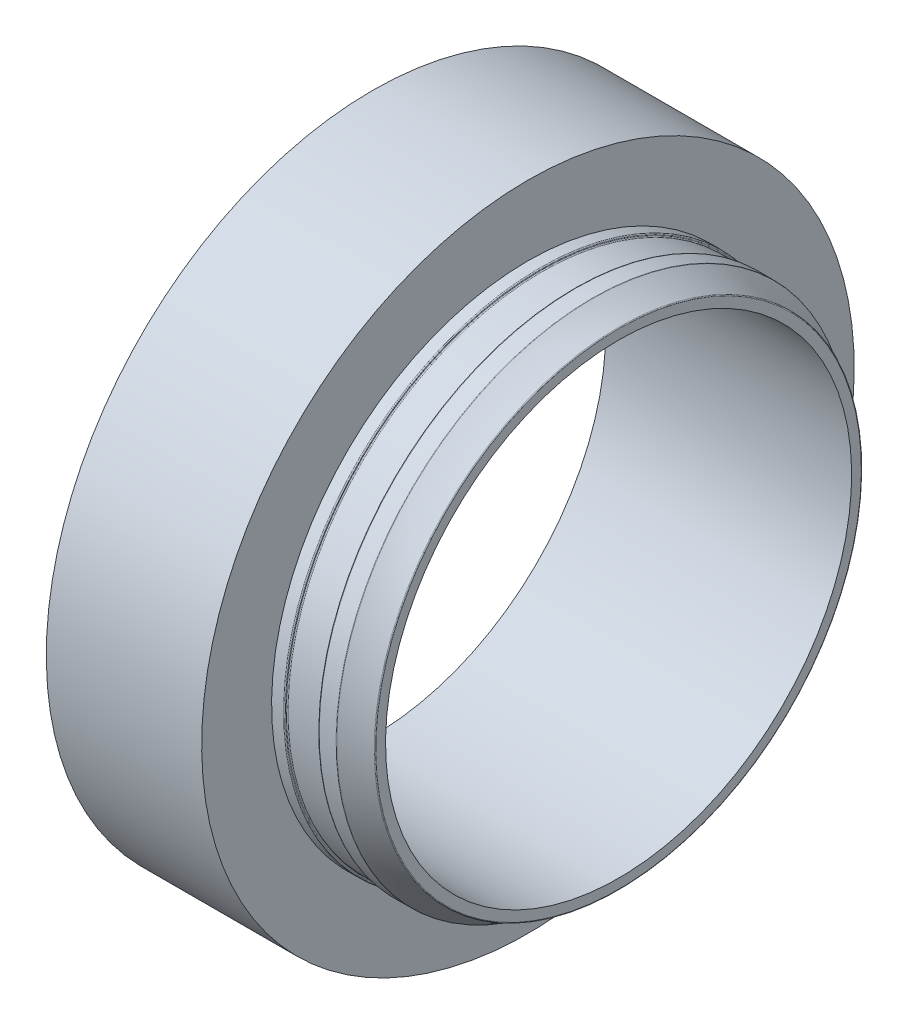
SolidWorks part; units mm, degrees
ref_plane "Front Plane" through (0, 0, 0) normal (0, 0, 1) x (1, 0, 0)
ref_plane "Top Plane" through (0, 0, 0) normal (0, 1, 0) x (1, 0, 0)
ref_plane "Right Plane" through (0, 0, 0) normal (1, 0, 0) x (0, 0, -1)
other "Configuration Table"
sketch "Sketch2" plane through (0, 0, 0) normal (0, 0, 1) x (1, 0, 0)
  line L0 (362.3463, 0) -> (0, 0) construction
  line L1 (169.4399, 49.5) -> (166.1963, 49.5)
  line L2 (165.7963, 49) -> (159.6963, 49)
  line L3 (159.2963, 49.5) -> (156.9963, 49.5)
  line L4 (156.9963, 63) -> (126.9963, 63)
  line L5 (156.9963, 63) -> (156.9963, 49.5)
  line L6 (126.9963, 63) -> (126.9963, 45)
  line L7 (165.9963, 49.3) -> (165.9963, 49.2)
  line L8 (159.4963, 49.3) -> (159.4963, 49.2)
  line L9 (174.4963, 46.8643) -> (174.4963, 45)
  line L10 (126.9963, 45) -> (174.4963, 45)
  arc A0 (159.4963, 49.2) -> (159.6963, 49) centre (159.6963, 49.2) ccw
  arc A1 (166.1963, 49.5) -> (165.9963, 49.3) centre (166.1963, 49.3) ccw
  arc A2 (165.7963, 49) -> (165.9963, 49.2) centre (165.7963, 49.2) ccw
  arc A3 (159.4963, 49.3) -> (159.2963, 49.5) centre (159.2963, 49.3) ccw
  arc A4 (169.5442, 49.4706) -> (174.3706, 47.05) centre (186.3234, 76.9043) ccw
  arc A5 (169.5442, 49.4706) -> (169.4399, 49.5) centre (169.4399, 49.3) ccw
  arc A6 (174.4963, 46.8643) -> (174.3706, 47.05) centre (174.2963, 46.8643) ccw
revolve "Revolve1" add sketch "Sketch2" angle 360 about L0
